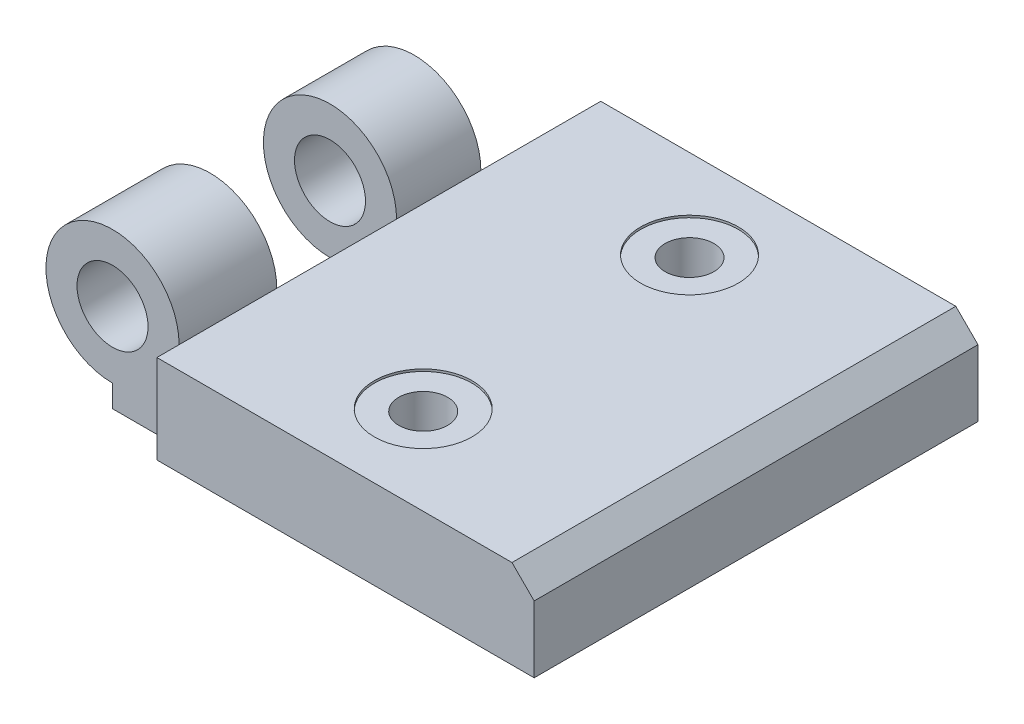
SolidWorks part; units mm, degrees
material "1060 合金"
ref_plane "前视基准面" through (0, 0, 0) normal (0, 0, 1) x (1, 0, 0)
ref_plane "上视基准面" through (0, 0, 0) normal (0, 1, 0) x (1, 0, 0)
ref_plane "右视基准面" through (0, 0, 0) normal (1, 0, 0) x (0, 0, -1)
sketch "草图1" plane through (0, 0, 0) normal (0, 0, 1) x (1, 0, 0)
  line L1 (-50, -10) -> (50, -10)
  line L2 (-50, -10) -> (-50, -5)
  line L3 (-35, 10) -> (50, 10)
  line L4 (50, -10) -> (50, 10)
  line L5 (-50, -10) -> (50, 10) construction
  line L6 (-35.2913, 7.0583) -> (50, -10) construction
  arc A0 (-35, 10) -> (-50, -5) centre (-50, 10) ccw
  point P0 (0, 0)
  dimension "D3" = 30
  dimension "D1" = 100
  dimension "D2" = 20
extrude "凸台-拉伸2" add sketch "草图1" along normal mid plane 100
sketch "草图2" plane through (0, 0, 50) normal (0, 0, 1) x (1, 0, 0)
  circle A0 centre (-50, 10) radius 8
  dimension "D1" = 16
extrude "切除-拉伸1" cut sketch "草图2" against normal through all both and the other way through all
sketch "草图3" plane through (0, 10, 0) normal (0, 1, 0) x (1, 0, 0)
  line L0 (-65, -50) -> (-35, -50) construction
  line L1 (-69.5676, -50) -> (-35, -50)
  line L2 (-69.5676, -23.0028) -> (-69.5676, 3.9972)
  line L3 (-69.1074, 50) -> (-35, 50)
  line L4 (-35, -23.0028) -> (-35, 3.9972)
  line L5 (-35, -50) -> (-35, 50) construction
  line L6 (-35, -50) -> (-69.5676, -50)
  line L7 (-35, -50) -> (-35, -45)
  line L8 (-35, -45) -> (-69.5676, -45)
  line L9 (-69.5676, 3.9972) -> (-35, 3.9972)
  line L10 (-69.5676, 22.9972) -> (-35, 22.9972)
  line L14 (-69.5676, -23.0028) -> (-35, -23.0028)
  line L15 (-35, 22.9972) -> (-35, 50)
  line L16 (-69.5676, -50) -> (-69.5676, -45)
  line L19 (-69.5676, 22.9972) -> (-69.1074, 50)
  point P0 (-49.8069, 3.9972)
  line M9 (-35, 50) -> (-35, -50)
  dimension "D1" = 27
  dimension "D2" = 19
  dimension "D3" = 27
  dimension "D4" = 5
extrude "切除-拉伸8" cut sketch "草图3" against normal through all both and the other way through all contours L19 L10 L3 M9 | L4 L9 L2 L14 | L7 L6 L16 L8
chamfer "倒角1" distance 5 angle 45 1 edges at (50, 10, 0)
sketch "草图4" plane through (0, 10, 0) normal (0, 1, 0) x (1, 0, 0)
  line L0 (5, 50) -> (5, 0) construction
  line L1 (45, 50) -> (-35, 50) construction
hole_wizard "M10 六角头螺栓的柱形沉头孔1" positions "3D草图1" profile "草图5" counterbore size "M10" standard "GB"
sketch3d "3D草图1"
  line L0 (5, 10, -50) -> (5, 10, 0) construction
  point P0 (5, 10, -25)
  point P5 (5, 10, -30)
  dimension "D1" = 30
sketch "草图5" plane through (5, 10, -30) normal (1, 0, 0) x (0, 0, 1)
  line L0 (0, 0) -> (0, 20.001)
  line L1 (0, 20.001) -> (5.5, 20.001)
  line L3 (5.5, 20.001) -> (5.5, 0.5)
  line L4 (5.5, 0.5) -> (11, 0.5)
  line L5 (11, 0.5) -> (11, 0)
  line L7 (11, 0) -> (0, 0)
  line L11 (0, -6.35) -> (0, 107.95) construction
  dimension "通孔孔直径" = 11
  dimension "通孔孔深度" = 20.001
  dimension "柱形沉头孔直径" = 22
  dimension "柱形沉头孔深度" = 0.5
mirror "镜向1" about plane through (0, 0, 0) normal (0, 0, 1) of "M10 六角头螺栓的柱形沉头孔1"
sketch "草图6" plane through (0, 10, 0) normal (0, 1, 0) x (1, 0, 0)
  line L0 (5, 30) -> (5, -30) construction
sketch "草图7" plane through (0, 10, 0) normal (0, 1, 0) x (1, 0, 0)
  line L0 (5, 50) -> (5, 30) construction
sketch "草图8" plane through (0, 10, 0) normal (0, 1, 0) x (1, 0, 0)
  line L0 (5, 30) -> (50, 30) construction
  line L1 (50, 50) -> (50, -50) construction
